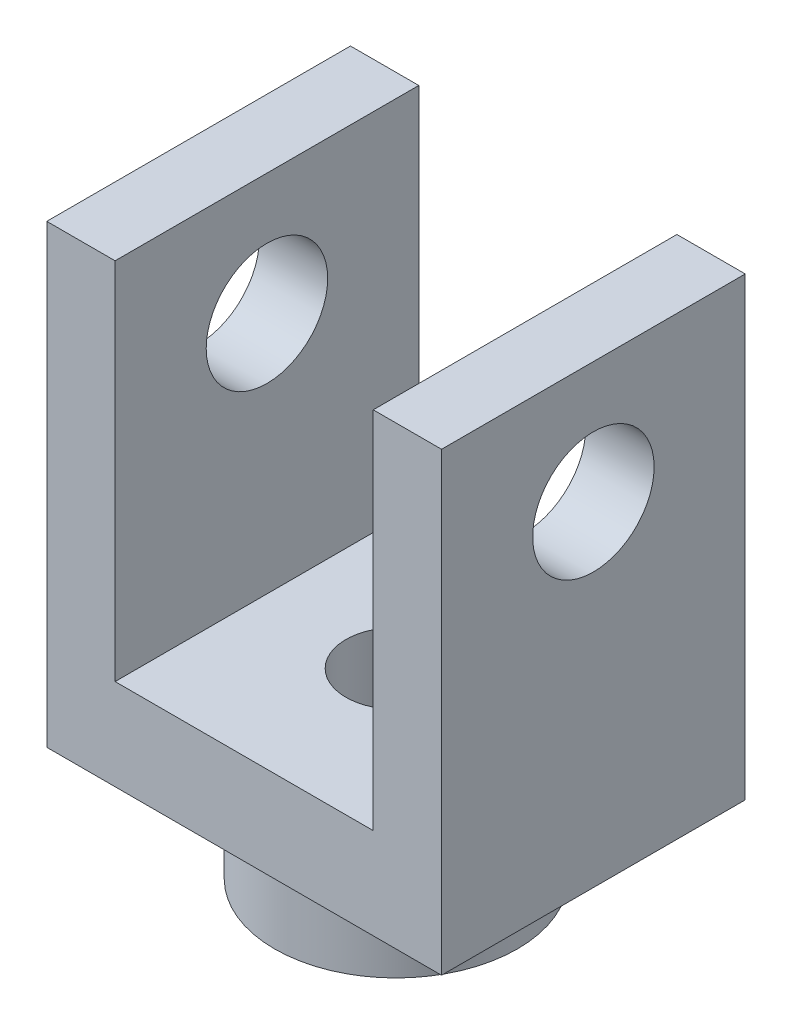
SolidWorks part; units mm, degrees
ref_plane "前视基准面" through (0, 0, 0) normal (0, 0, 1) x (1, 0, 0)
ref_plane "上视基准面" through (0, 0, 0) normal (0, 1, 0) x (1, 0, 0)
ref_plane "右视基准面" through (0, 0, 0) normal (1, 0, 0) x (0, 0, -1)
sketch "草图1" plane through (0, 0, 0) normal (0, 0, 1) x (1, 0, 0)
  line L1 (6.5, -7.5) -> (-6.5, -7.5)
  line L2 (6.5, -7.5) -> (6.5, 7.5)
  line L3 (6.5, 7.5) -> (-6.5, 7.5)
  line L4 (-6.5, -7.5) -> (-6.5, 7.5)
  line L5 (6.5, -7.5) -> (-6.5, 7.5) construction
  line L6 (6.5, 7.5) -> (-6.5, -7.5) construction
  point P0 (0, 0)
  dimension "D1" = 13
  dimension "D2" = 15
extrude "凸台-拉伸1" add sketch "草图1" along normal mid plane 10
sketch "草图2" plane through (0, 0, 5) normal (0, 0, 1) x (1, 0, 0)
  line L0 (6.5, 7.5) -> (-6.5, 7.5) construction
  line L1 (4.25, 19.5) -> (-4.25, 19.5)
  line L2 (4.25, 19.5) -> (4.25, -4.5)
  line L3 (4.25, -4.5) -> (-4.25, -4.5)
  line L4 (-4.25, 19.5) -> (-4.25, -4.5)
  line L5 (4.25, 19.5) -> (-4.25, -4.5) construction
  line L6 (4.25, -4.5) -> (-4.25, 19.5) construction
  point P0 (0, 7.5)
  dimension "D1" = 8.5
  dimension "D2" = 12
extrude "切除-拉伸1" cut sketch "草图2" against normal blind 10
sketch "草图3" plane through (6.5, 0, 0) normal (1, 0, 0) x (0, 0, -1)
  line L0 (0, 7.5) -> (0, 3.5) construction
  line L1 (-5, 7.5) -> (5, 7.5) construction
  circle A0 centre (0, 3.5) radius 2
  dimension "D1" = 4
  dimension "D2" = 4
extrude "切除-拉伸2" cut sketch "草图3" against normal blind 25
sketch "草图11" plane through (0, -7.5, 0) normal (0, -1, 0) x (1, 0, 0)
  circle A0 centre (0, 0) radius 2
  dimension "D1" = 4
sketch "草图13" plane through (0, -7.5, 0) normal (0, -1, 0) x (1, 0, 0)
  circle A0 centre (0, 0) radius 4
  dimension "D1" = 8
extrude "凸台-拉伸2" add sketch "草图13" along normal blind 3
hole_wizard "M4x0.7 螺纹孔1" positions "3D草图2" profile "草图12" tap size "M4x0.7" standard "BSI"
sketch3d "3D草图2"
  line L0 (0, -10.5, 0) -> (0, -7.5, 0) construction
  point P6 (0, -10.5, 0)
sketch "草图12" plane through (0, -10.5, 0) normal (1, 0, 0) x (0, 0, -1)
  line L0 (0, 0) -> (0, 11.0914)
  line L1 (0, 11.0914) -> (1.65, 10.1)
  line L2 (1.65, 10.1) -> (1.65, 0)
  line L5 (1.65, 0) -> (0, 0)
  line L10 (0, 11.0914) -> (-1.65, 10.1) construction
  line L11 (0, -6.35) -> (0, 107.95) construction
  dimension "螺纹孔钻头直径" = 3.3
  dimension "螺纹孔钻头深度" = 10.1
  dimension "导头角度" = 118
cosmetic thread "孔螺蚊线1" parameters "D1"=6, "D2"=4
